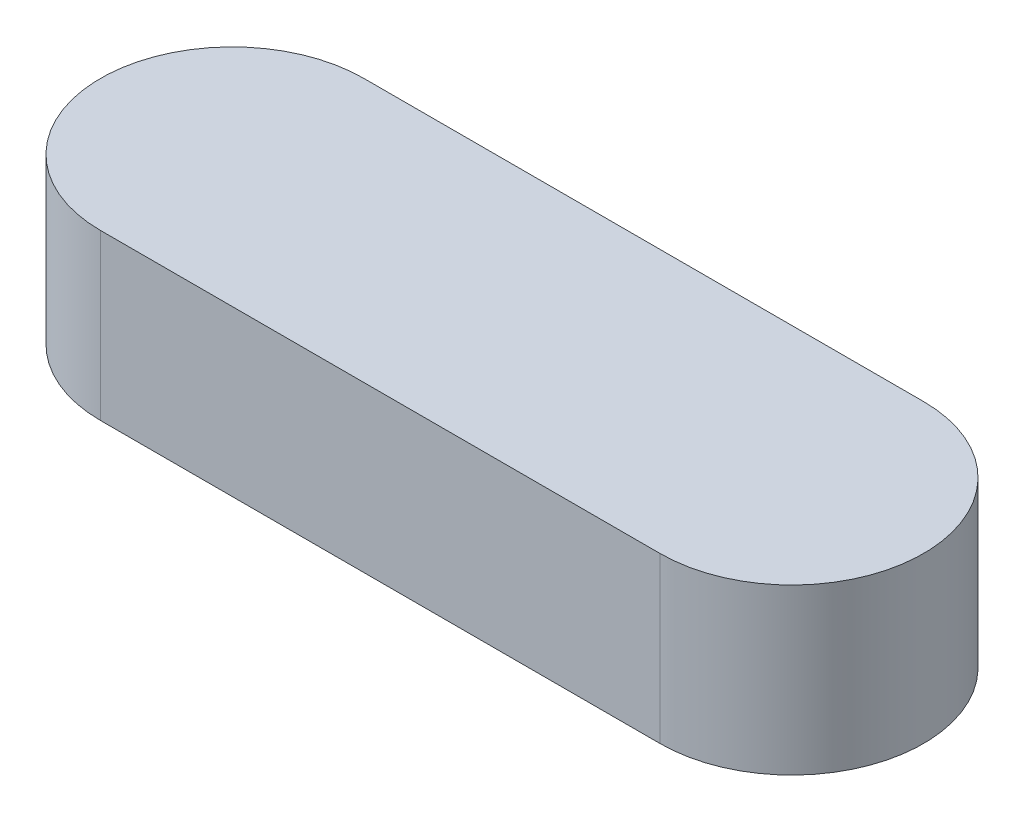
SolidWorks part; units mm, degrees
ref_plane "Front Plane" through (0, 0, 0) normal (0, 0, 1) x (1, 0, 0)
ref_plane "Top Plane" through (0, 0, 0) normal (0, 1, 0) x (1, 0, 0)
ref_plane "Right Plane" through (0, 0, 0) normal (1, 0, 0) x (0, 0, -1)
sketch "Sketch1" plane through (0, 0, 0) normal (0, 1, 0) x (1, 0, 0)
  line L0 (0, 0) -> (34, 0) construction
  line L1 (0, 8) -> (34, 8)
  line L2 (0, -8) -> (34, -8)
  arc A0 (0, 8) -> (0, -8) centre (0, 0) ccw
  arc A1 (34, -8) -> (34, 8) centre (34, 0) ccw
  point P3 (17, 0)
  point P8 (-8, 0)
  point P9 (42, 0)
extrude "Boss-Extrude1" add sketch "Sketch1" along normal blind 10
equation "\"b\"= 16"
equation "\"h\"= 10"
equation "\"l\"= 50"
equation "\"D1@Sketch1\"=\"b\"/2"
equation "\"D2@Sketch1\"=\"l\""
equation "\"D1@Boss-Extrude1\"=\"h\""
